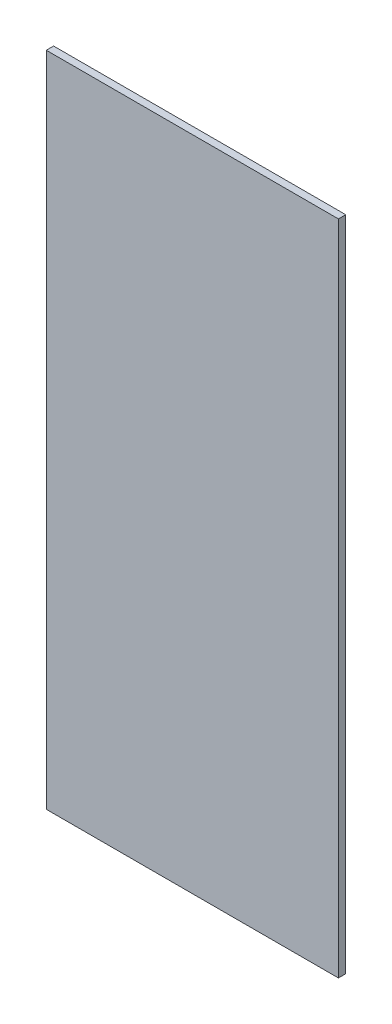
from build123d import *

# Parameters (mm, degrees)
SKETCH_1_W      = 800
SKETCH_1_H      = 1800
EXTRUDE_1_DEPTH = 20


with BuildPart() as part:
    # 草图1 → 凸台-拉伸1 (new body)
    with BuildSketch(Plane.XY):
        Rectangle(SKETCH_1_W, SKETCH_1_H)
    extrude(amount=EXTRUDE_1_DEPTH)


solid = part.part
